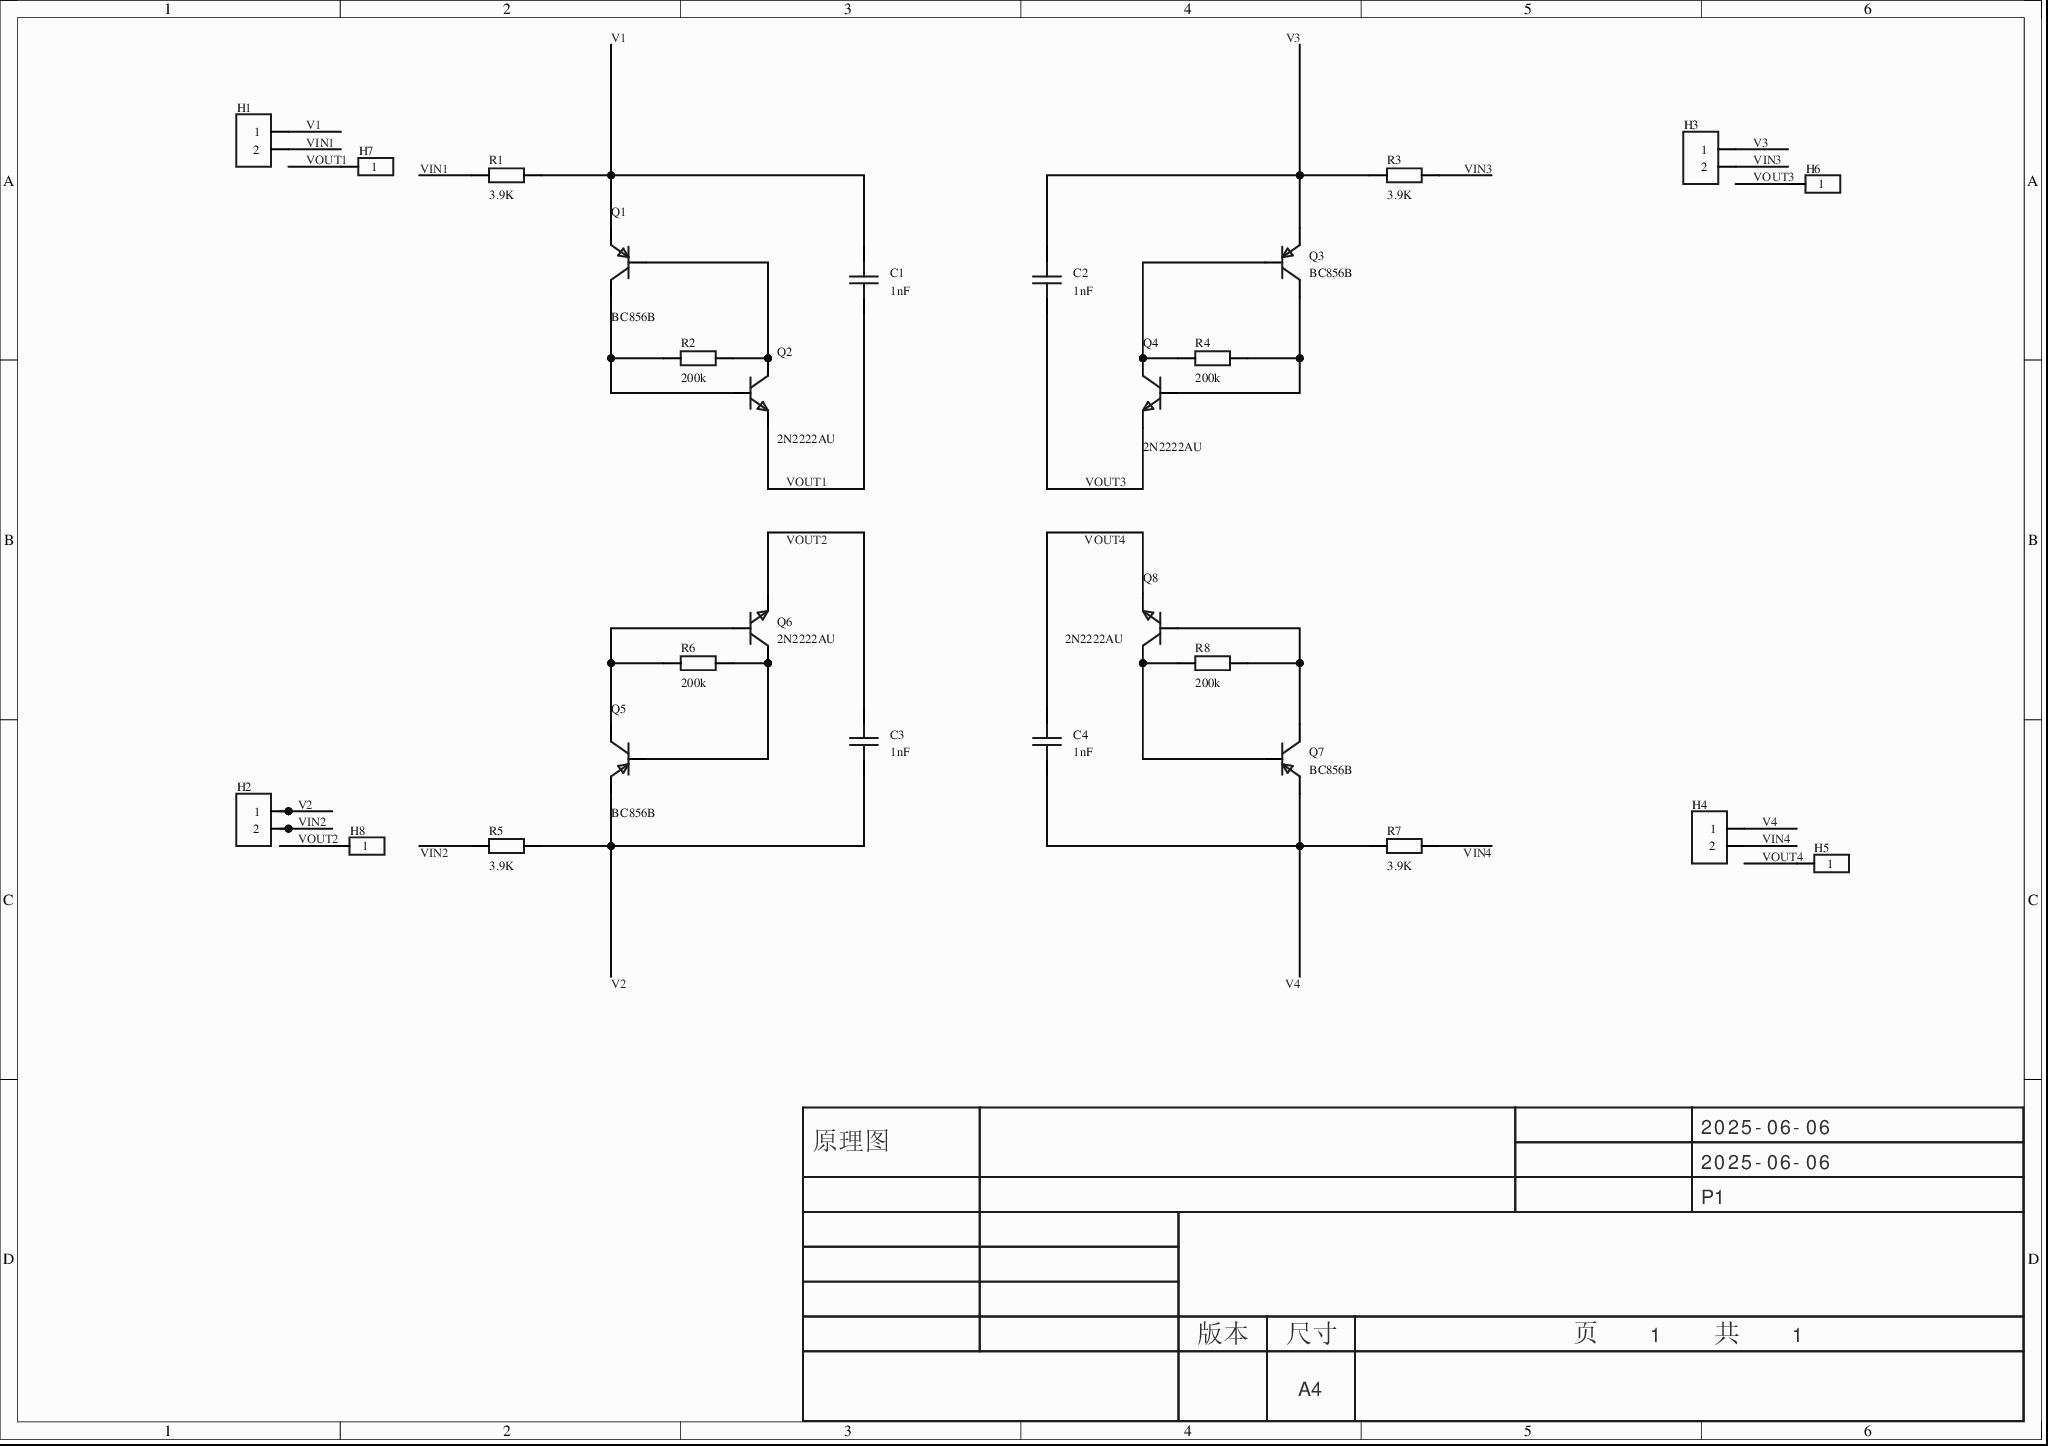
[diagram p0: MISC51349-3.schdoc]
# Altium project MISC51349-2.PrjPcb
1 sheet, 28 parts. Net scope: global (net labels, ports and power ports of the same name join across sheets).
Board file: MISC51349.pcbdoc

## Sheet MISC51349-3.schdoc
size 297 x 209 mm; Version: V1.0; @Project Name: MISC51349; @Page Count: 1; @Update Date: 2025-06-06; @Create Date: 2025-06-06; @Schematic Name: MISC51349; @Page No: 1; @Create Time: 22:09:27; @Update Time: 22:39:39; @Board Name: MISC51349

### Parts
C1  1nF  [C0402]
C2  1nF  [C0402]
C3  1nF  [C0402]
C4  1nF  [C0402]
H1  (no value)  [HDR-TH_2P-P2.54-V-F]
H2  (no value)  [HDR-TH_2P-P2.54-V-F]
H3  (no value)  [HDR-TH_2P-P2.54-V-F]
H4  (no value)  [HDR-TH_2P-P2.54-V-F]
H5  (no value)  [HDR-TH_1P-V-M_XKB_X4611WV-01I-C28D40]
H6  (no value)  [HDR-TH_1P-V-M_XKB_X4611WV-01I-C28D40]
H7  (no value)  [HDR-TH_1P-V-M_XKB_X4611WV-01I-C28D40]
H8  (no value)  [HDR-TH_1P-V-M_XKB_X4611WV-01I-C28D40]
Q1  BC856B  [SOT-23-3_L2.9-W1.6-P1.90-LS2.8-BR]
Q2  2N2222AU  [SOT-89-3_L4.5-W2.4-P1.50-LS4.0-BR]
Q3  BC856B  [SOT-23-3_L2.9-W1.6-P1.90-LS2.8-BR]
Q4  2N2222AU  [SOT-89-3_L4.5-W2.4-P1.50-LS4.0-BR]
Q5  BC856B  [SOT-23-3_L2.9-W1.6-P1.90-LS2.8-BR]
Q6  2N2222AU  [SOT-89-3_L4.5-W2.4-P1.50-LS4.0-BR]
Q7  BC856B  [SOT-23-3_L2.9-W1.6-P1.90-LS2.8-BR]
Q8  2N2222AU  [SOT-89-3_L4.5-W2.4-P1.50-LS4.0-BR]
R1  3.9K  [R0402]
R2  200k  [R0402]
R3  3.9K  [R0402]
R4  200k  [R0402]
R5  3.9K  [R0402]
R6  200k  [R0402]
R7  3.9K  [R0402]
R8  200k  [R0402]

### Nets
V1: C1.2 H1.1 Q1.2(E) R1.2
V2: C3.2 H2.1 Q5.2(E) R5.2
V3: C2.2 H3.1 Q3.2(E) R3.2
V4: C4.2 H4.1 Q7.2(E) R7.2
VIN1: H1.2 R1.1
VIN2: H2.2 R5.1
VIN3: H3.2 R3.1
VIN4: H4.2 R7.1
VOUT1: C1.1 H7.1 Q2.2
VOUT2: C3.1 H8.1 Q6.2
VOUT3: C2.1 H6.1 Q4.2
VOUT4: C4.1 H5.1 Q8.2
NetQ1_1: Q1.1(B) Q2.3 R2.2
NetQ1_3: Q1.3(C) Q2.1 R2.1
NetQ3_1: Q3.1(B) Q4.3 R4.2
NetQ3_3: Q3.3(C) Q4.1 R4.1
NetQ5_1: Q5.1(B) Q6.3 R6.2
NetQ5_3: Q5.3(C) Q6.1 R6.1
NetQ7_1: Q7.1(B) Q8.3 R8.2
NetQ7_3: Q7.3(C) Q8.1 R8.1

### Notes on the sheet
- 2025-06-06
- 原理图
- P1
- 版本
- 尺寸
- A4
- 页    1    共    1

### Library data of the parts
C1-C4 = CAP_0402: ConvertToPcb: yes; SymbolName: CapAcitance; ModelId: 36a51122f27c49738f86b3bfa98863e0; ModelName: C0402_L1.0-W0.5-H0.5; ModelTransform: 39.37,19.685,0,0,0,0,0,0,0; Value: 1nF; Device: CAP_0402; AddInBom: yes; Supplier Footprint: 0402; FootprintName: C0402
H1-H4 = HDR-F_2.54_1x2P: Symbol: Header-Female-2.54_1x2; ConvertToPcb: yes; ModelId: a9450ef445564560a104363b9aacde4e; ModelName: HDR-TH_2P-P2.54-F-LI-1X2P; ModelTransform: 215.7476,98.425,0,0,0,0,0,0,-129.921; Device: HDR-F_2.54_1x2P; AddInBom: yes; SupplierPart: C49661; Supplier Footprint: 插件; FootprintName: HDR-TH_2P-P2.54-V-F
H5-H8 = HDR-M_2.54_1x1P: Symbol: HDR_1x1; ConvertToPcb: yes; ModelId: 95857080d3cc4057a19a22ccce05e171; ModelTransform: 78.74,79.1337,0,0,0,0,0,0,-110.236; Device: HDR-M_2.54_1x1P; AddInBom: yes; SupplierPart: C81276; Supplier Footprint: 插件; FootprintName: HDR-TH_1P-V-M_XKB_X4611WV-01I-C28D40; JLCPCB Part Class: Extended Part; ModelName: HDR-TH_1P-V-M_XKB_X4611WV-01I-C28D40
Q1 Q3 Q5 Q7 = BC856B_C181144: 晶体管类型:PNP;集电极电流(Ic):100mA;集射极击穿电压(Vceo):65V;耗散功率(Pd):200mW;直流电流增益(hFE):220@2mA,5V;; Manufacturer: Hottech(合科泰); AddInBom: yes; ModelId: 89cb27a44ab2466697082bb9fd73a7d0; ModelName: SOT-23-3L_L2.9-W1.6-H1.1-LS2.8-P0.95; ModelTransform: 114.173,110.236,0,90,0,0,0,0,0; type: PNP; Current - Collector(Ic): 100mA; Collector - Emitter Voltage VCEO: 65V; Pd - Power Dissipation: 200mW; Transition frequency(fT): 100MHz; Current - Collector Cutoff: 100nA; Vce Saturation(VCE(sat)): 500mV; Symbol: BC856B_C181144; Device: BC856B_C181144; LCSC Part Name: BC856B; SupplierPart: C181144; ManufacturerPart: BC856B; Supplier Footprint: SOT-23; JLCPCB Part Class: 扩展库; Datasheet: https://atta.szlcsc.com/upload/public/pdf/source/20220506/36890928A961043A8557960C54EC9FEA.pdf; Supplier: LCSC; ConvertToPcb: yes; FootprintName: SOT-23-3_L2.9-W1.6-P1.90-LS2.8-BR; DC Current Gain: 220@2mA,5V; Operating Temperature: -
Q2 Q4 Q6 Q8 = 2N2222AU: Manufacturer: CBI(创基); AddInBom: yes; ModelId: dde435042bae4b9691e74da94cf9d9f3; ModelTransform: 177.165,161.417,0,90,0,0,-2.323,0,0; Symbol: 2N2222AU; Device: 2N2222AU; LCSC Part Name: 2N2222AU; SupplierPart: C21714170; ManufacturerPart: 2N2222AU; Supplier Footprint: SOT-89; JLCPCB Part Class: 扩展库; Datasheet: https://atta.szlcsc.com/upload/public/pdf/source/20240307/3DBBF7265193D2D4CDAA5BD73FF82DD6.pdf; Supplier: LCSC; ConvertToPcb: yes; FootprintName: SOT-89-3_L4.5-W2.4-P1.50-LS4.0-BR; ModelName: SOT-89-3_L4.5-W2.4-P1.50-LS4.0-BR
R1-R8 = Res_0402: Symbol: 电阻; ConvertToPcb: yes; ModelId: 671aefced39d4c318694bba8bd8efd39; ModelName: R0402_L1.0-W0.5-H0.5; ModelTransform: 39.37,19.685,0,0,0,0,0,0.0005,0; Device: Res_0402; AddInBom: yes; Supplier Footprint: 0402; FootprintName: R0402
  R1 R3 R5 R7: Value: 3.9K
  R2 R4 R6 R8: Value: 200k